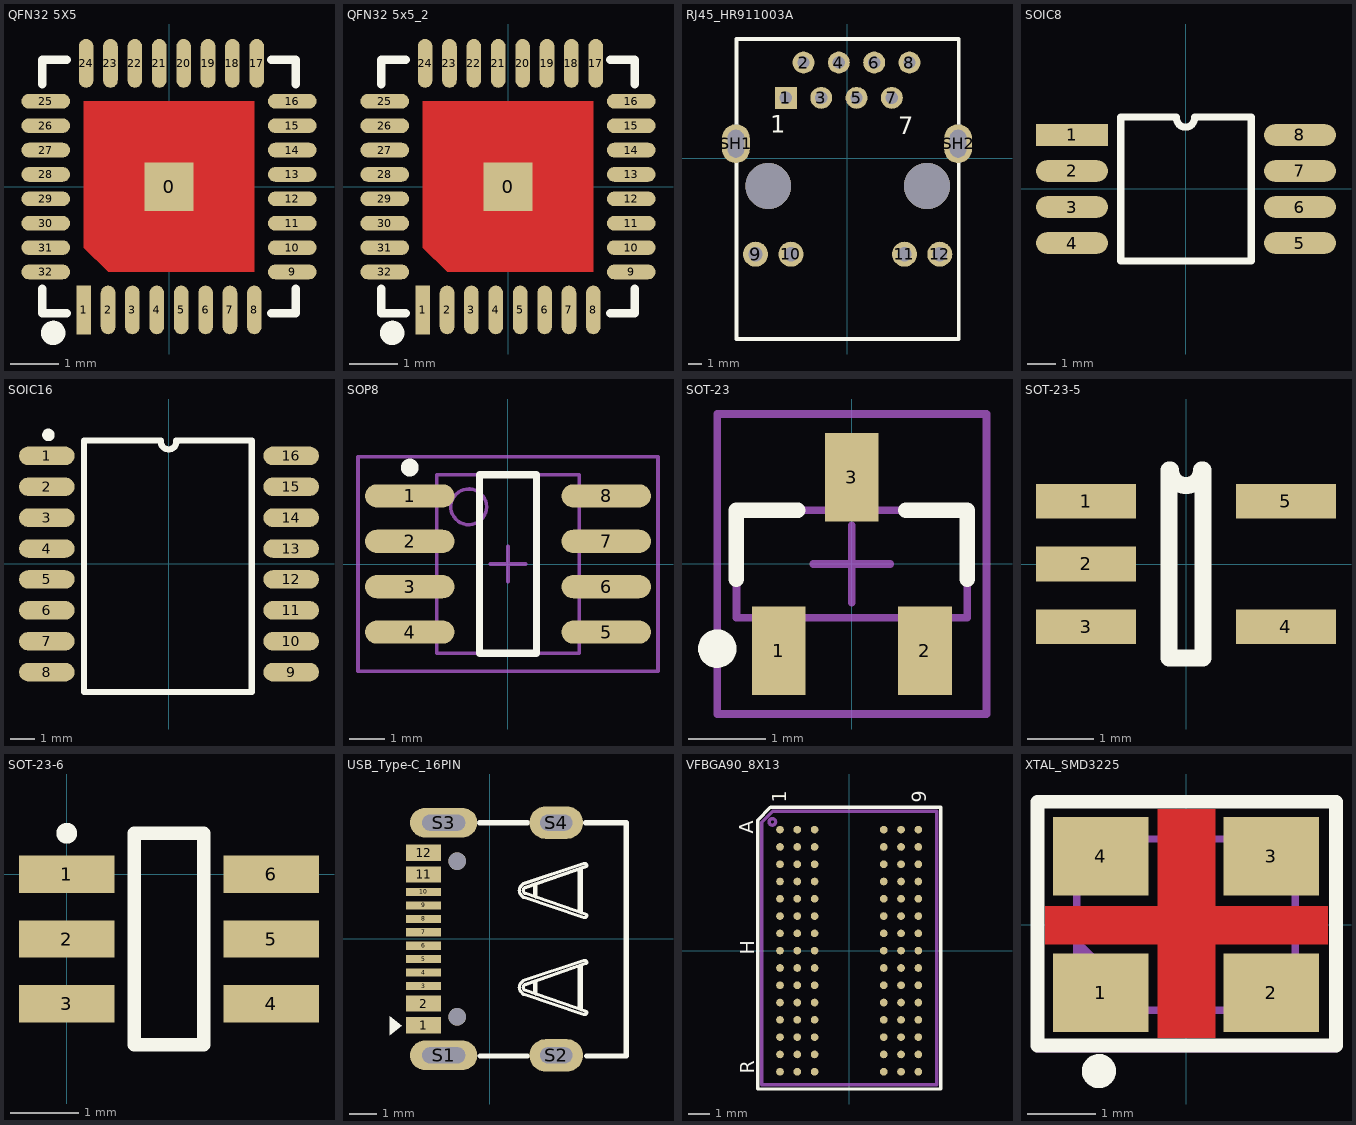
[diagram p0: the footprints below, top view; thin cyan lines are the x and y axes]
# Altium footprint library MISC105414-6.PcbLib: 28 footprints (part 2 of 2)
Each footprint in its own frame and in the unit in brackets; x right, y up, seen from the top. Pads: shape width x height; smd on the part's side, far side on the other; paste and mask are expansions set on the pad; w line width, h text height; cw(c..) or ccw(c..) is an arc to the next point about the centre after c.

## QFN32 5X5 [mm]
pads (33):
  rect 1x1 smd: 0(0,0)
  rect 0.3x1 smd: 1(-1.751,-2.528)
  oval 0.3x1 smd: 2(-1.25,-2.528) 3(-0.75,-2.528) 4(-0.25,-2.528) 5(0.25,-2.528) 6(0.75,-2.528) 7(1.25,-2.528) 8(1.75,-2.528) 17(1.8,2.528) 18(1.3,2.528) 19(0.8,2.528) 20(0.3,2.528) 21(-0.2,2.528) 22(-0.7,2.528) 23(-1.2,2.528) 24(-1.7,2.528)
  oval 1x0.3 smd: 9(2.528,-1.75) 10(2.528,-1.25) 11(2.528,-0.75) 12(2.528,-0.25) 13(2.528,0.25) 14(2.528,0.75) 15(2.528,1.25) 16(2.528,1.75) 25(-2.528,1.75) 26(-2.528,1.25) 27(-2.528,0.75) 28(-2.528,0.25) 29(-2.528,-0.25) 30(-2.528,-0.75) 31(-2.528,-1.25) 32(-2.528,-1.75)
Top Layer:
  region: -1.75,1.75 1.75,1.75 1.75,-1.75 -1.25,-1.75 -1.75,-1.25
Top Overlay:
  circle w0.25: c-2.375,-3 r0.125
  lines w0.178: -2.6,-2.1 -2.6,-2.6 -2.1,-2.6 ; -2.6,2.1 -2.6,2.6 -2.1,2.6 ; 2.1,-2.6 2.6,-2.6 2.6,-2.1 ; 2.1,2.6 2.6,2.6 2.6,2.1
Mechanical 15:
  circle w0.05: c0,0 r0.35
  lines w0.05: -0.5,0 0.5,0 ; 0,-0.5 0,0.5
3D body "QFN32 5x5.STEP": height 0.93, standoff 0, extent -2.475,-2.526 2.527,2.476

## QFN32 5x5_2 [mm]
pads (33):
  rect 1x1 smd: 0(0,0)
  rect 0.3x1 smd: 1(-1.751,-2.528)
  oval 0.3x1 smd: 2(-1.25,-2.528) 3(-0.75,-2.528) 4(-0.25,-2.528) 5(0.25,-2.528) 6(0.75,-2.528) 7(1.25,-2.528) 8(1.75,-2.528) 17(1.8,2.528) 18(1.3,2.528) 19(0.8,2.528) 20(0.3,2.528) 21(-0.2,2.528) 22(-0.7,2.528) 23(-1.2,2.528) 24(-1.7,2.528)
  oval 1x0.3 smd: 9(2.528,-1.75) 10(2.528,-1.25) 11(2.528,-0.75) 12(2.528,-0.25) 13(2.528,0.25) 14(2.528,0.75) 15(2.528,1.25) 16(2.528,1.75) 25(-2.528,1.75) 26(-2.528,1.25) 27(-2.528,0.75) 28(-2.528,0.25) 29(-2.528,-0.25) 30(-2.528,-0.75) 31(-2.528,-1.25) 32(-2.528,-1.75)
Top Layer:
  region: -1.75,1.75 1.75,1.75 1.75,-1.75 -1.25,-1.75 -1.75,-1.25
Top Overlay:
  circle w0.25: c-2.375,-3 r0.125
  lines w0.178: -2.6,-2.1 -2.6,-2.6 -2.1,-2.6 ; -2.6,2.1 -2.6,2.6 -2.1,2.6 ; 2.1,-2.6 2.6,-2.6 2.6,-2.1 ; 2.1,2.6 2.6,2.6 2.6,2.1
Mechanical 15:
  circle w0.05: c0,0 r0.35
  lines w0.05: -0.5,0 0.5,0 ; 0,-0.5 0,0.5
3D body "QFN32 5x5.STEP": height 0.93, standoff 0, extent -2.475,-2.526 2.527,2.476

## RJ45_HR911003A [mm] "HR911003A"
pads (14):
  rect 1.575x1.575 hole 0.889: 1(-4.395,4.355)
  round 1.575 hole 0.889: 2(-3.125,6.895) 3(-1.855,4.355) 4(-0.585,6.895) 5(0.685,4.355) 6(1.955,6.895) 7(3.225,4.355) 8(4.495,6.895)
  round 1.8 hole 1.02: 9(-6.575,-6.895) 10(-4.035,-6.895) 11(4.135,-6.895) 12(6.675,-6.895)
  oval 2x2.8 hole 1.2 slot 2 at 90 deg: SH1(-7.995,1.055) SH2(7.995,1.055)
via -5.665,-1.995 diameter 3.3 hole 3.3
via 5.765,-1.995 diameter 3.3 hole 3.3
Top Overlay:
  lines w0.254: -7.95,-12.995 -7.95,8.588 8.05,8.588 8.05,-12.995 -7.95,-12.995
  text "1" at -5.531,1.826 h1.27
  text "7" at 3.687,1.74 h1.27

## SOIC8 [mil]
pads (8):
  rect 100x30 smd: 1(-158.31,75)
  oval 100x30 smd: 2(-158.31,25) 3(-158.31,-25) 4(-158.31,-75) 5(158.31,-75) 6(158.31,-25) 7(158.31,25) 8(158.31,75)
Top Overlay:
  lines w10: -13.19,98.43 ccw(c-0.69,98.43) 11.81,98.43 ; -13.19,100 -90.55,100 -90.55,-100 90.55,-100 90.55,100 11.81,100
3D body "User Library-SOIC-8-1.step": height 68.94, standoff -0.05, extent -118.04,-96.46 118.21,96.45

## SOIC16 [mil]
pads (16):
  oval 90x30 smd: 1(-197.83,175) 2(-197.83,125) 3(-197.83,75) 4(-197.83,25) 5(-197.83,-25) 6(-197.83,-75) 7(-197.83,-125) 8(-197.83,-175) 9(197.84,-175) 10(197.84,-125) 11(197.84,-75) 12(197.84,-25) 13(197.84,25) 14(197.84,75) 15(197.84,125) 16(197.84,175)
Top Overlay:
  circle w12: c-195.19,209.02 r4.12
  lines w10: -13.19,198.03 ccw(c-0.69,198.03) 11.81,198.03 ; -13.19,200 -137.76,200 -137.76,-207.48 133.9,-207.48 133.9,200 11.81,200

## SOP8 [mm]
pads (8):
  oval 2.5x0.65 smd: 1(-2.75,1.905) 2(-2.75,0.635) 3(-2.75,-0.635) 4(-2.75,-1.905) 5(2.75,-1.905) 6(2.75,-0.635) 7(2.75,0.635) 8(2.75,1.905)
Top Overlay:
  circle w0.25: c-2.75,2.7 r0.125
  lines w0.2: -0.8,-2.5 -0.8,2.5 0.8,2.5 0.8,-2.5 -0.8,-2.5
Mechanical 13:
  circle w0.1: c-1.1,1.6 r0.5
  lines w0.1: -2,-2.5 -2,2.5 2,2.5 2,-2.5 -2,-2.5
Mechanical 15:
  lines w0.1: -0.5,0 0.5,0 ; 0,-0.5 0,0.5 ; -4.2,-3 -4.2,3 4.2,3 4.2,-3 -4.2,-3
3D body: height 1.75, standoff 0, extent -2,-2.5 2,2.5

## SOT-23 [mm]
pads (3):
  rect 0.7x1.15 smd: 1(-0.95,-1.125) 2(0.95,-1.125) 3(0,1.125)
Top Overlay:
  circle w0.25: c-1.75,-1.1 r0.125
  lines w0.2: -1.5,-0.2 -1.5,0.7 -0.7,0.7 ; 0.7,0.7 1.5,0.7 1.5,-0.2
Mechanical 13:
  lines w0.1: -1.5,-0.7 1.5,-0.7 1.5,0.7 -1.5,0.7 -1.5,-0.7
Mechanical 15:
  lines w0.1: -0.5,0 0.5,0 ; 0,-0.5 0,0.5 ; -1.75,-1.95 1.75,-1.95 1.75,1.95 -1.75,1.95 -1.75,-1.95
3D body: height 1.1, standoff 0, extent -1.5,-0.7 1.5,0.7

## SOT-23-5 [mm]
pads (5):
  rect 1.5x0.52 smd: 1(-1.497,0.94) 2(-1.497,0) 3(-1.497,-0.94) 4(1.497,-0.94) 5(1.497,0.94)
Top Overlay:
  lines w0.254: -0.254,1.41 -0.254,-1.41 0.254,-1.41 0.254,1.41 ; -0.235,1.41 ccw(c0,1.41) 0.235,1.41
3D body "SOT-23-5.STEP": height 1.2, standoff 0, extent -1.451,-1.425 1.349,1.475

## SOT-23-6 [mm]
pads (6):
  rect 1.4x0.55 smd: 1(0,0) 2(0,-0.95) 3(0,-1.9) 4(3,-1.9) 5(3,-0.95) 6(3,0)
Top Overlay:
  circle w0.254: c0,0.6 r0.025
  lines w0.2: 0.992,-2.5 2.008,-2.5 2.008,0.6 0.992,0.6 0.992,-2.5
3D body "SOT23-6.STEP": height 1.15, standoff -0.03, extent 0,-2.45 2.807,0.55

## USB_Type-C_16PIN [mm]
pads (18):
  rect 1.3x0.6 smd mask+0.064: 1(-2.463,-3.2) 2(-2.463,-2.4) 11(-2.463,2.4) 12(-2.463,3.2)
  rect 1.3x0.3 smd mask+0.064: 3(-2.463,-1.75) 4(-2.463,-1.25) 5(-2.463,-0.75) 6(-2.463,-0.25) 7(-2.463,0.25) 8(-2.463,0.75) 9(-2.463,1.25) 10(-2.463,1.75)
  oval 2.5x1.1 hole 0.6 slot 1.6 at 0 deg: S1(-1.717,-4.32) S3(-1.717,4.32)
  oval 2x1.2 hole 0.6 slot 1.2 at 0 deg: S2(2.462,-4.32) S4(2.462,4.32)
  round 0.65 hole 0.65 unplated mask+0: ""(-1.218,-2.89) ""(-1.218,2.89)
Top Overlay:
  region: -3.275,-3.225 -3.725,-2.875 -3.725,-3.575
  lines w0.12: 1.665,-2.023 1.665,-1.573 ; 1.665,1.577 1.665,2.027 ; 1.715,-2.048 1.715,-1.548 ; 1.715,1.552 1.715,2.052 ; 3.315,-2.598 3.315,-0.998 ; 3.315,1.002 3.315,2.602 ; 3.39,-2.623 3.39,-0.973 ; 3.39,0.977 3.39,2.627 ; 1.275,-1.713 ccw(c1.361,-1.798) 1.24,-1.798 ccw(c1.361,-1.798) 1.275,-1.883 1.29,-1.898 3.59,-2.698 cw(c3.515,-2.723) 3.49,-2.798 1.24,-2.048 1.161,-1.969 cw(c1.331,-1.798) 1.09,-1.798 cw(c1.331,-1.798) 1.161,-1.627 1.24,-1.548 3.49,-0.798 cw(c3.515,-0.873) 3.59,-0.898 1.29,-1.698 ; 1.275,-1.713 1.29,-1.698 ; 1.275,-1.713 1.29,-1.698 ; 1.275,1.717 cw(c1.361,1.802) 1.24,1.802 cw(c1.361,1.802) 1.275,1.887 1.29,1.902 3.59,2.702 ccw(c3.515,2.727) 3.49,2.802 1.24,2.052 1.161,1.973 ccw(c1.331,1.802) 1.09,1.802 ccw(c1.331,1.802) 1.161,1.631 1.24,1.552 3.49,0.802 ccw(c3.515,0.877) 3.59,0.902 1.29,1.702 ; 1.275,1.717 1.29,1.702 ; 1.275,1.717 1.29,1.702
  lines w0.2: -0.373,4.32 1.382,4.32 ; -0.37,-4.343 1.385,-4.343 ; 3.563,4.32 5.066,4.32 5.066,-4.343 3.593,-4.343
3D body "User Library-USB Type C Port (SMD Type).STEP": height 3.2, standoff -1, extent -2.86,-4.47 5.041,4.47

## VFBGA90_8X13 [mil]
pads (90):
  round 14 smd: A1(-125.98,220.46) A2(-94.49,220.46) A3(-62.99,220.46) A7(62.99,220.46) A8(94.49,220.46) A9(125.98,220.46) B1(-125.98,188.97) B2(-94.49,188.97) B3(-62.99,188.97) B7(62.99,188.97) B8(94.49,188.97) B9(125.98,188.97) C1(-125.98,157.47) C2(-94.49,157.47) C3(-62.99,157.47) C7(62.99,157.47) C8(94.49,157.47) C9(125.98,157.47) D1(-125.98,125.98) D2(-94.49,125.98) D3(-62.99,125.98) D7(62.99,125.98) D8(94.49,125.98) D9(125.98,125.98) E1(-125.98,94.48) E2(-94.49,94.48) E3(-62.99,94.48) E7(62.99,94.48) E8(94.49,94.48) E9(125.98,94.48) F1(-125.98,62.98) F2(-94.49,62.98) F3(-62.99,62.98) F7(62.99,62.98) F8(94.49,62.98) F9(125.98,62.98) G1(-125.98,31.49) G2(-94.49,31.49) G3(-62.99,31.49) G7(62.99,31.49) G8(94.49,31.49) G9(125.98,31.49) H1(-125.98,-0.01) H2(-94.49,-0.01) H3(-62.99,-0.01) H7(62.99,-0.01) H8(94.49,-0.01) H9(125.98,-0.01) J1(-125.98,-31.5) J2(-94.49,-31.5) J3(-62.99,-31.5) J7(62.99,-31.5) J8(94.49,-31.5) J9(125.98,-31.5) K1(-125.98,-62.99) K2(-94.49,-62.99) K3(-62.99,-62.99) K7(62.99,-62.99) K8(94.49,-62.99) K9(125.98,-62.99) L1(-125.98,-94.49) L2(-94.49,-94.49) L3(-62.99,-94.49) L7(62.99,-94.49) L8(94.49,-94.49) L9(125.98,-94.49) M1(-125.98,-125.99) M2(-94.49,-125.99) M3(-62.99,-125.99) M7(62.99,-125.99) M8(94.49,-125.99) M9(125.98,-125.99) N1(-125.98,-157.48) N2(-94.49,-157.48) N3(-62.99,-157.48) N7(62.99,-157.48) N8(94.49,-157.48) N9(125.98,-157.48) P1(-125.98,-188.98) P2(-94.49,-188.98) P3(-62.99,-188.98) P7(62.99,-188.98) P8(94.49,-188.98) P9(125.98,-188.98) R1(-125.98,-220.47) R2(-94.49,-220.47) R3(-62.99,-220.47) R7(62.99,-220.47) R8(94.49,-220.47) R9(125.98,-220.47)
Top Overlay:
  lines w5.98: -166.54,-251.97 166.54,-251.97 166.54,261.02 -143.46,261.02 -166.54,237.94 -166.54,-251.97
  text "R" at -173.23,-224.41 h25
  text "H" at -173.23,-7.88 h25
  text "A" at -174.5,213.42 h25
  text "1" at -115,269.49 h25
  text "9" at 140,269.49 h25
Mechanical 16:
  circle w6: c-140,234.49 r6
  lines w5.98: -159.45,-244.09 159.45,-244.09 159.45,253.93 -139.45,253.93 -159.45,233.93 -159.45,-244.09
3D body: height 150, standoff 0, extent -159.45,-244.09 159.45,253.94

## XTAL_SMD3225 [mm]
pads (4):
  rect 1.4x1.15 smd: 1(-1.25,-1) 2(1.25,-1) 3(1.25,1) 4(-1.25,1)
Top Layer:
  pour cut-out: -2.062,-0.292 -2.062,0.266 2.078,0.266 2.078,-0.292
  pour cut-out: -0.411,-1.664 -0.411,1.689 0.427,1.689 0.427,-1.664
Top Overlay:
  circle w0.25: c-1.277,-2.15 r0.125
  lines w0.203: -2.177,-1.775 2.198,-1.775 2.198,1.8 -2.177,1.8 -2.177,-1.775
Mechanical 15:
  lines w0.1: -1.6,-1.15 -1.5,-1.25 ; -1.6,-1.05 -1.4,-1.25 ; -1.6,-0.95 -1.3,-1.25 ; -1.6,-0.85 -1.2,-1.25 ; -1.6,-0.75 -1.1,-1.25 ; -1.6,-0.65 -1,-1.25 ; -1.6,-0.55 -0.9,-1.25 ; -1.6,-0.45 -0.8,-1.25 ; -1.6,-0.35 -0.7,-1.25 ; -1.6,-0.25 -0.6,-1.25 ; -1.6,-1.25 1.6,-1.25 1.6,1.25 -1.6,1.25 -1.6,-1.25
Mechanical 16:
  circle w0.05: c0,0 r0.35
  lines w0.001: -1.65,-1.3 1.65,-1.3 1.65,1.3 -1.65,1.3 -1.65,-1.3
  lines w0.05: -0.5,0 0.5,0 ; 0,-0.5 0,0.5 ; -2.2,-1.85 2.2,-1.85 2.2,1.85 -2.2,1.85 -2.2,-1.85